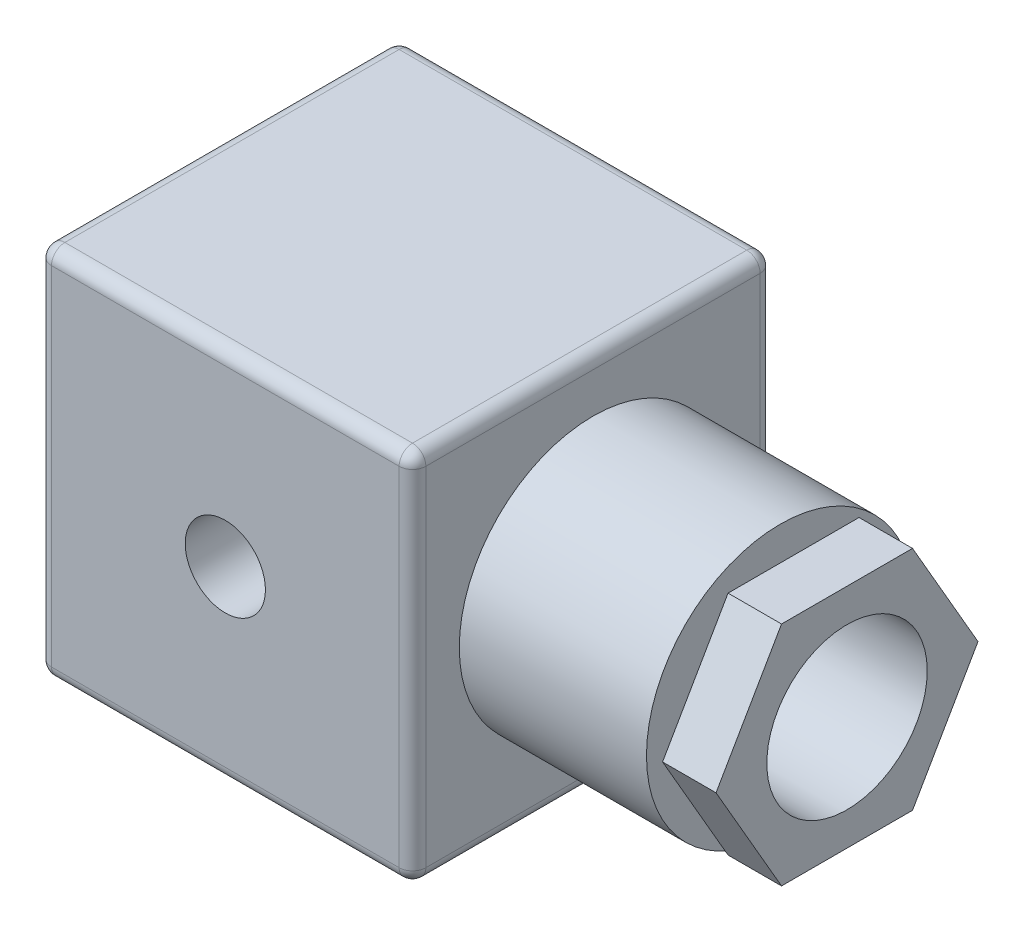
from build123d import *

# Parameters (mm, degrees)
SKETCH1_W           = 28
SKETCH1_H           = 28
SKETCH1_W_2         = 0.581812165
SKETCH1_H_2         = 3.033734858
BOSS_EXTRUDE1_DEPTH = 27
SKETCH2_W           = 28
SKETCH2_H           = 28
BOSS_EXTRUDE2_DEPTH = 2
SKETCH3_R           = 3
CUT_EXTRUDE1_DEPTH  = 6
SKETCH4_R           = 1.5
CUT_EXTRUDE2_DEPTH  = 25
FILLET1_R           = 1
SKETCH5_R           = 10
SKETCH5_R_2         = 5
EXTRUDE_THIN1_DEPTH = 15
BOSS_EXTRUDE3_DEPTH = 4
CUT_EXTRUDE3_START  = -1
SKETCH7_R           = 10
SKETCH7_R_2         = 7
CUT_EXTRUDE3_DEPTH  = 1
SKETCH8_R           = 6
CUT_EXTRUDE4_DEPTH  = 22
SKETCH9_W           = 8.469861182
SKETCH9_H           = 8.944508274
CUT_EXTRUDE5_DEPTH  = 15


with BuildPart() as part:
    # Sketch1 → Boss-Extrude1 (new body)
    with BuildSketch(Plane.XY):
        with Locations((17, 0)):
            Rectangle(SKETCH1_W, SKETCH1_H)
        Polygon((18.5, 7.071580399), (18.5, 6.29199588), (18.76385967, 6.29199588), (18.76385967, 6.681788139), (21.23614033, 6.681788139), (21.23614033, 6.29199588), (21.5, 6.29199588), (21.5, 7.071580399), align=None, mode=Mode.SUBTRACT)
        with Locations((10.815679405, 0)):
            Rectangle(SKETCH1_W_2, SKETCH1_H_2, mode=Mode.SUBTRACT)
        Polygon((18.5, -6.29199588), (18.5, -7.071580399), (21.5, -7.071580399), (21.5, -6.29199588), (21.23614033, -6.29199588), (21.23614033, -6.681788139), (18.76385967, -6.681788139), (18.76385967, -6.29199588), align=None, mode=Mode.SUBTRACT)
    extrude(amount=BOSS_EXTRUDE1_DEPTH)

    # Sketch2 → Boss-Extrude2 (add)
    with BuildSketch(Plane.XY.offset(27)):
        with Locations((17, 0)):
            Rectangle(SKETCH2_W, SKETCH2_H)
    extrude(amount=-BOSS_EXTRUDE2_DEPTH)

    # Sketch3 → Cut-Extrude1 (cut)
    with BuildSketch(Plane.XY.offset(27)):
        with Locations((17, 0)):
            Circle(SKETCH3_R)
    extrude(amount=-CUT_EXTRUDE1_DEPTH, mode=Mode.SUBTRACT)

    # Sketch4 → Cut-Extrude2 (cut)
    with BuildSketch(Plane.XY.offset(21)):
        with Locations((17, 0)):
            Circle(SKETCH4_R)
    extrude(amount=-CUT_EXTRUDE2_DEPTH, mode=Mode.SUBTRACT)

    # Fillet1
    fillet1_edges = [part.edges().sort_by_distance(p)[0] for p in [
        (3, 0, 27),
        (17, -14, 27),
        (31, 0, 27),
        (17, -14, 0),
        (3, 0, 0),
        (17, 14, 0),
        (31, 0, 0),
        (31, -14, 13.5),
        (3, -14, 13.5),
        (3, 14, 13.5),
        (31, 14, 13.5),
        (17, 14, 27),
    ]]
    fillet(fillet1_edges, radius=FILLET1_R)

    # Sketch5 → Extrude-Thin1 (add)
    with BuildSketch(Plane(origin=(31, 0, 0), x_dir=(0, 0, -1), z_dir=(1, 0, 0))):
        with Locations((-13.5, 0)):
            Circle(SKETCH5_R)
        with Locations((-13.5, 0)):
            Circle(SKETCH5_R_2, mode=Mode.SUBTRACT)
    extrude(amount=EXTRUDE_THIN1_DEPTH)

    # Sketch6 → Boss-Extrude3 (add)
    with BuildSketch(Plane(origin=(46, 0, 0), x_dir=(0, 0, -1), z_dir=(1, 0, 0))):
        Polygon((-23.296433781, 0), (-18.398216891, -8.483960521), (-8.601783109, -8.483960521), (-3.703566219, 0), (-8.601783109, 8.483960521), (-18.398216891, 8.483960521), align=None)
    extrude(amount=BOSS_EXTRUDE3_DEPTH)

    # Sketch7 → Cut-Extrude3 (cut)
    with BuildSketch(Plane(origin=(46, 0, 0), x_dir=(0, 0, -1), z_dir=(1, 0, 0)).offset(CUT_EXTRUDE3_START)):
        with Locations(Location((-13.5, 0, 0), (0, 0, 270))):
            Circle(SKETCH7_R)
        with Locations(Location((-13.5, 0, 0), (0, 0, 90))):
            Circle(SKETCH7_R_2, mode=Mode.SUBTRACT)
    extrude(amount=CUT_EXTRUDE3_DEPTH, mode=Mode.SUBTRACT)

    # Sketch8 → Cut-Extrude4 (cut)
    with BuildSketch(Plane(origin=(50, 0, 0), x_dir=(0, 0, -1), z_dir=(1, 0, 0))):
        with Locations((-13.5, 0)):
            Circle(SKETCH8_R)
    extrude(amount=-CUT_EXTRUDE4_DEPTH, mode=Mode.SUBTRACT)

    # Sketch9 → Cut-Extrude5 (cut)
    with BuildSketch(Plane(origin=(0, 0, 0), x_dir=(-1, 0, 0), z_dir=(0, 0, -1))):
        with Locations((-17, 0)):
            Rectangle(SKETCH9_W, SKETCH9_H)
    extrude(amount=-CUT_EXTRUDE5_DEPTH, mode=Mode.SUBTRACT)


solid = part.part
